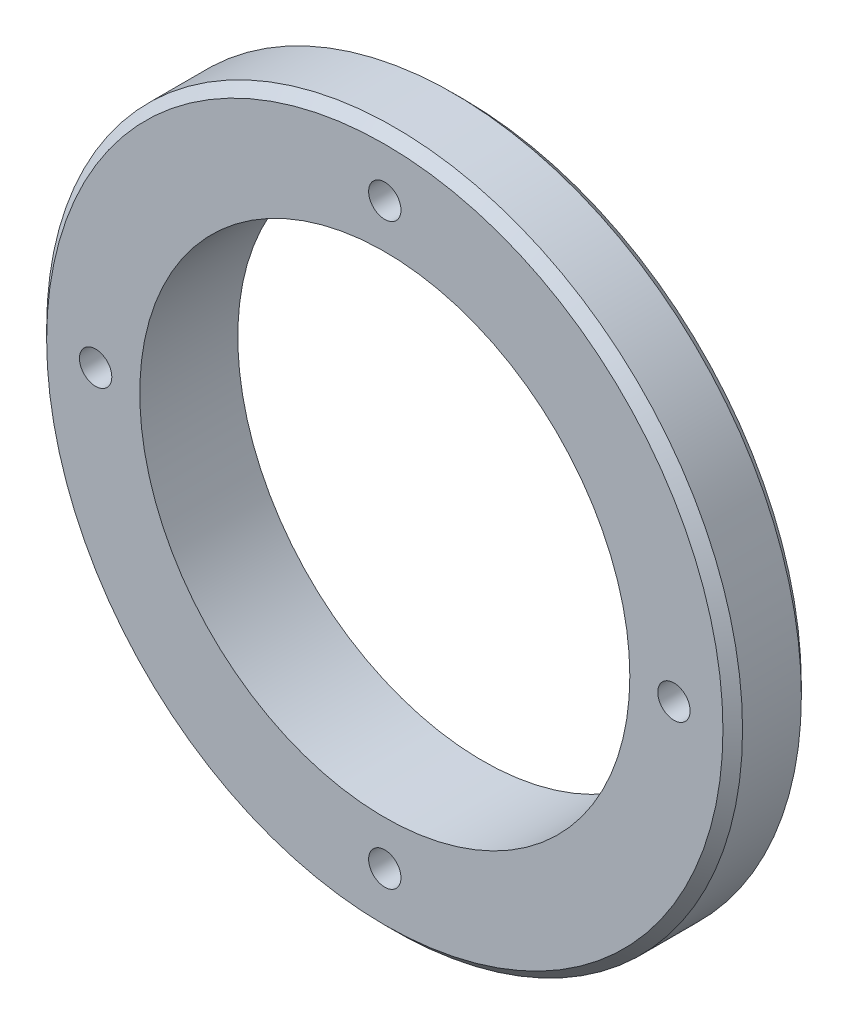
from build123d import *

# Parameters (mm, degrees)
SKETCH1_R           = 35.5
SKETCH1_R_2         = 25
BOSS_EXTRUDE1_DEPTH = 10
SKETCH2_R           = 1.25
CUT_EXTRUDE1_DEPTH  = 52.190819489
SKETCH3_R           = 35.5
SKETCH3_R_2         = 26.5
CUT_EXTRUDE2_DEPTH  = 2
M4_TAPPED_HOLE1_D   = 3.3
CHAMFER1_SIZE       = 1


with BuildPart() as part:
    # Sketch1 → Boss-Extrude1 (new body)
    with BuildSketch(Plane.XY):
        Circle(SKETCH1_R)
        Circle(SKETCH1_R_2, mode=Mode.SUBTRACT)
    extrude(amount=BOSS_EXTRUDE1_DEPTH)

    # Sketch2 → Cut-Extrude1 (cut, through all)
    with BuildSketch(Plane.XY.offset(10)):
        with Locations((0, 29.5)):
            Circle(SKETCH2_R)
        with Locations((29.5, 0)):
            Circle(SKETCH2_R)
        with Locations((0, -29.5)):
            Circle(SKETCH2_R)
        with Locations((-29.5, 0)):
            Circle(SKETCH2_R)
    extrude(amount=-CUT_EXTRUDE1_DEPTH, mode=Mode.SUBTRACT)

    # Sketch3 → Cut-Extrude2 (cut)
    with BuildSketch(Plane(origin=(0, 0, 0), x_dir=(-1, 0, 0), z_dir=(0, 0, -1))):
        Circle(SKETCH3_R)
        Circle(SKETCH3_R_2, mode=Mode.SUBTRACT)
    extrude(amount=-CUT_EXTRUDE2_DEPTH, mode=Mode.SUBTRACT)

    # M4 Tapped Hole1 (through all)
    with Locations(Plane.XY.offset(10)):
        with Locations((0, -29.5), (-29.5, 0), (0, 29.5), (29.5, 0)):
            Hole(M4_TAPPED_HOLE1_D / 2)

    # Chamfer1
    chamfer1_edges = [part.edges().sort_by_distance(p)[0] for p in [
        (-35.5, 0, 2),
        (-35.5, 0, 10),
    ]]
    chamfer(chamfer1_edges, length=CHAMFER1_SIZE)


solid = part.part
